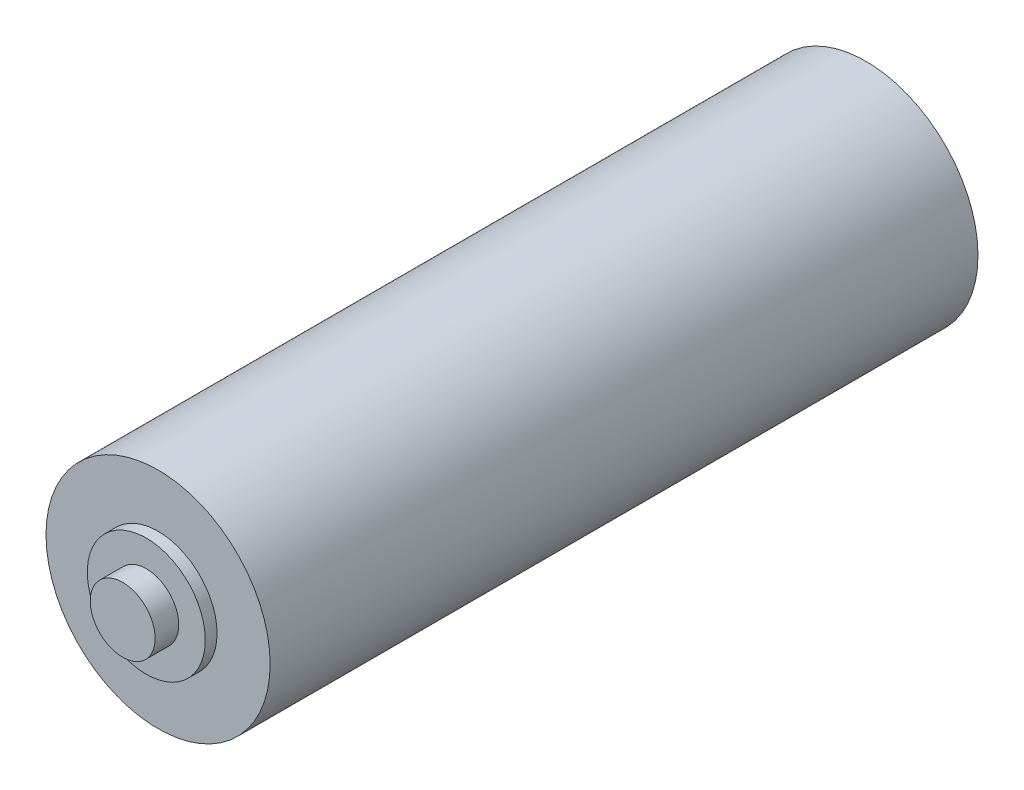
from build123d import *

# Parameters (mm, degrees)
SKETCH1_R           = 95
BOSS_EXTRUDE1_DEPTH = 600
SKETCH2_R           = 50
BOSS_EXTRUDE2_DEPTH = 10
BOSS_EXTRUDE3_START = 10
SKETCH3_R           = 50
BOSS_EXTRUDE3_DEPTH = 10
SKETCH4_R           = 27.5
BOSS_EXTRUDE4_DEPTH = 20
BOSS_EXTRUDE5_START = 20
SKETCH5_R           = 27.5
BOSS_EXTRUDE5_DEPTH = 20


with BuildPart() as part:
    # Sketch1 → Boss-Extrude1 (new body)
    with BuildSketch(Plane.XY):
        Circle(SKETCH1_R)
    extrude(amount=BOSS_EXTRUDE1_DEPTH)

    # Sketch2 → Boss-Extrude2 (add)
    with BuildSketch(Plane.XY.offset(600)):
        Circle(SKETCH2_R)
    extrude(amount=BOSS_EXTRUDE2_DEPTH)

    # Sketch3 → Boss-Extrude3 (add)
    with BuildSketch(Plane(origin=(0, 0, 0), x_dir=(-1, 0, 0), z_dir=(0, 0, -1)).offset(BOSS_EXTRUDE3_START)):
        with Locations(Location((0, 0, 0), (0, 0, 180))):
            Circle(SKETCH3_R)
    extrude(amount=-BOSS_EXTRUDE3_DEPTH)

    # Sketch4 → Boss-Extrude4 (add)
    with BuildSketch(Plane(origin=(0, 0, -10), x_dir=(-1, 0, 0), z_dir=(0, 0, -1))):
        Circle(SKETCH4_R)
    extrude(amount=BOSS_EXTRUDE4_DEPTH)

    # Sketch5 → Boss-Extrude5 (add)
    with BuildSketch(Plane.XY.offset(610).offset(BOSS_EXTRUDE5_START)):
        with Locations(Location((0, 0, 0), (0, 0, 180))):
            Circle(SKETCH5_R)
    extrude(amount=-BOSS_EXTRUDE5_DEPTH)


solid = part.part
